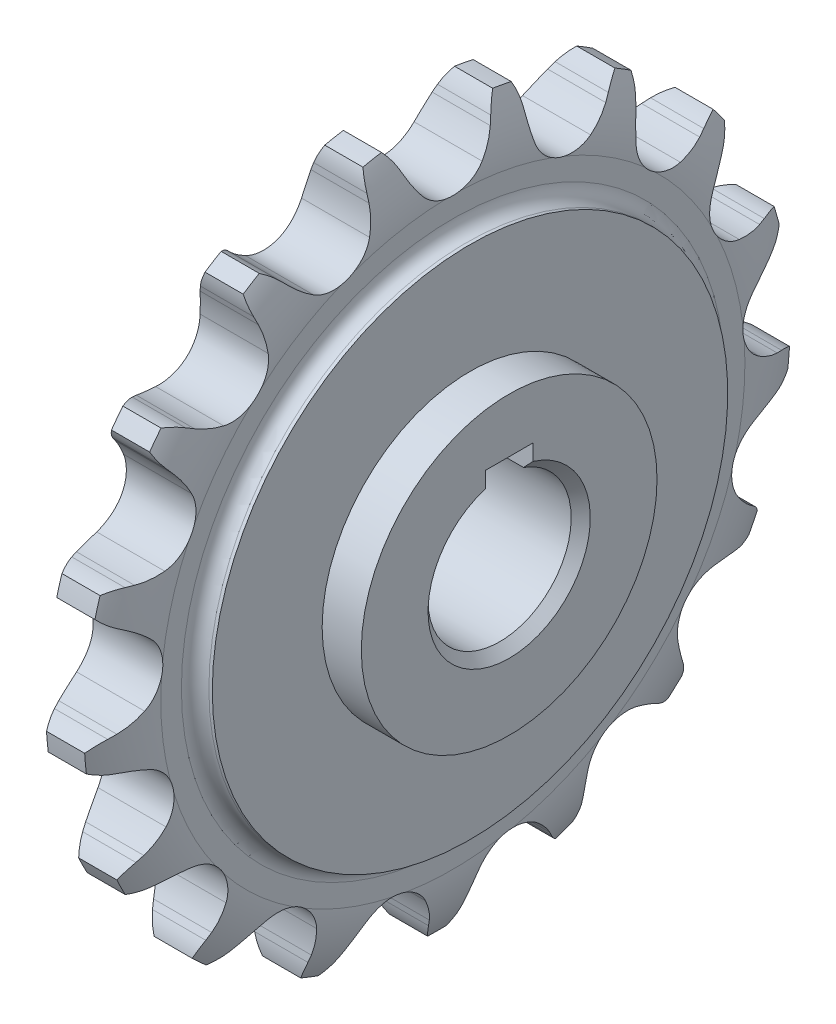
SolidWorks part; units mm, degrees
ref_plane "前视基准面" through (0, 0, 0) normal (0, 0, 1) x (1, 0, 0)
ref_plane "上视基准面" through (0, 0, 0) normal (0, 1, 0) x (1, 0, 0)
ref_plane "右视基准面" through (0, 0, 0) normal (1, 0, 0) x (0, 0, -1)
sketch "草图1" plane through (0, 0, 0) normal (0, 0, 1) x (1, 0, 0)
  line L0 (-6.35, 0) -> (6.35, 0) construction
  line L1 (-5.4492, 7.5) -> (-5.4492, 27)
  line L2 (-5.4492, 27) -> (-5.0894, 27)
  line L3 (-3.6503, 28.4392) -> (-3.6502, 30.5979)
  line L4 (-1.9992, 37) -> (1.9992, 37)
  line L5 (3.6502, 30.5979) -> (3.6503, 28.4392)
  line L6 (5.0894, 27) -> (5.4492, 27)
  line L7 (5.4492, 27) -> (5.4492, 7.5)
  line L8 (5.4492, 7.5) -> (-5.4492, 7.5)
  line L9 (0, 0) -> (0, 37) construction
  line L10 (-3.0626, 34.5579) -> (3.0626, 34.5579) construction
  line L11 (-3.0626, -34.5579) -> (3.0626, -34.5579) construction
  line L12 (6.35, 0) -> (23.35, 0) construction
  line L13 (-3.6502, 30.5979) -> (3.7984, 30.5979) construction
  line L14 (-3.6502, -30.5979) -> (3.7984, -30.5979) construction
  line L15 (23.35, 0) -> (31.27, 0) construction
  line L16 (31.27, 0) -> (43.34, 0) construction
  line L17 (43.34, 0) -> (51.19, 0) construction
  line L18 (51.19, 0) -> (65.57, 0) construction
  arc A0 (-1.9992, 37) -> (-3.6502, 30.5979) centre (9.049, 30.7369) ccw
  arc A1 (1.9992, 37) -> (3.6502, 30.5979) centre (-9.049, 30.7369) cw
  arc A2 (3.6503, 28.4392) -> (5.0894, 27) centre (5.0894, 28.4392) ccw
  arc A3 (-5.0894, 27) -> (-3.6503, 28.4392) centre (-5.0894, 28.4392) ccw
  point P30 (3.6502, 27)
  point P33 (-3.6502, 27)
  dimension "D1" = 3.5979
  dimension "rx" = 12.7
  dimension "D3" = 1.4392
  dimension "d" = 69.1158
  dimension "p" = 12.7
  dimension "z" = 17
  dimension "da" = 74
  dimension "df" = 61.1958
  dimension "dr" = 7.92
  dimension "dk" = 15
  dimension "dg" = 54
  dimension "h" = 12.07
  dimension "bf1" = 7.3005
  dimension "b1" = 7.85
  dimension "ba" = 1.651
  dimension "D2" = 1.799
  dimension "pt" = 14.38
revolve "旋转1" add sketch "草图1" angle 360 about L0
sketch "草图2" plane through (0, 0, 0) normal (1, 0, 0) x (0, 0, -1)
  line L0 (0, 0) -> (0, 37) construction
  line L1 (0, 0) -> (-6.7987, 36.37) construction
  line L2 (0, 0) -> (-13.3659, 34.5015) construction
  line L3 (3.1525, 32.0477) -> (1.2637, 33.5517) construction
  line L4 (4.526, 34.3177) -> (-4.9566, 38.5047) construction
  line L5 (0, 0) -> (6.7987, 36.37) construction
  line L6 (4.526, 34.3177) -> (4.8285, 35.0028)
  line L7 (-4.526, 34.3177) -> (-4.8285, 35.0028)
  circle A0 centre (0, 0) radius 37 construction
  arc A1 (3.1525, 32.0477) -> (-3.1525, 32.0477) centre (0, 34.5579) cw
  arc A2 (3.1525, 32.0477) -> (4.526, 34.3177) centre (-4.9566, 38.5047) ccw
  arc A3 (5.8231, 36.5389) -> (4.8285, 35.0028) centre (10.1207, 32.666) ccw
  arc A4 (-3.1525, 32.0477) -> (-4.526, 34.3177) centre (4.9566, 38.5047) cw
  arc A5 (-5.8231, 36.5389) -> (-4.8285, 35.0028) centre (-10.1207, 32.666) cw
  arc A7 (5.8231, 36.5389) -> (-5.8231, 36.5389) centre (0, 0) ccw
  dimension "r1" = 4.0298
  dimension "r3" = 5.7852
  dimension "D1" = 21.176
  dimension "D2" = 10.588
  dimension "α/2" = 51.471
  dimension "M" = 4.9566
  dimension "T" = 3.9468
  dimension "β" = 14.706
  dimension "γ/2" = 13.235
  dimension "bc" = 0.7488
extrude "切除-拉伸1" cut sketch "草图2" against normal mid plane 10.8984
pattern_circular "阵列(圆周)1" count 17 over 360 about axis through (0, 0, 0) along (1, 0, 0) of "切除-拉伸1"
sketch "草图3" plane through (0, 0, 0) normal (0, 0, 1) x (1, 0, 0)
  line L0 (5.4492, 7.5) -> (9.5508, 7.5)
  line L3 (9.5508, 7.5) -> (9.5508, 15.4912)
  line L4 (9.5508, 15.4912) -> (5.4492, 15.4912)
  line L5 (5.4492, 15.4912) -> (5.4492, 7.5)
  line L6 (0, 0) -> (4.8, 0) construction
  line L8 (-5.4492, 27) -> (-5.4492, -27) construction
  dimension "h" = 7.9912
  dimension "K" = 4.8
  dimension "L" = 15
revolve "旋转2" add sketch "草图3" angle 360 about L6
sketch "草图4" plane through (-5.4492, 0, 0) normal (-1, 0, 0) x (0, 0, 1)
  line L1 (-2.5, 7.0711) -> (2.5, 7.0711)
  line L2 (-2.5, 7.0711) -> (-2.5, 9.8)
  line L3 (-2.5, 9.8) -> (2.5, 9.8)
  line L4 (2.5, 7.0711) -> (2.5, 9.8)
  circle A0 centre (0, 0) radius 7.5 construction
  point P6 (0.2, 9.8)
  dimension "D1" = 9.8
  dimension "键槽宽度" = 5
  dimension "t1" = 2.3
extrude "切除-拉伸2" cut sketch "草图4" against normal through all
chamfer "倒角1" distance 1 angle 45 1 edges at (-5.4492, -7.5, 0)
chamfer "倒角3" distance 1 angle 45 1 edges at (9.5508, -7.5, 0)
